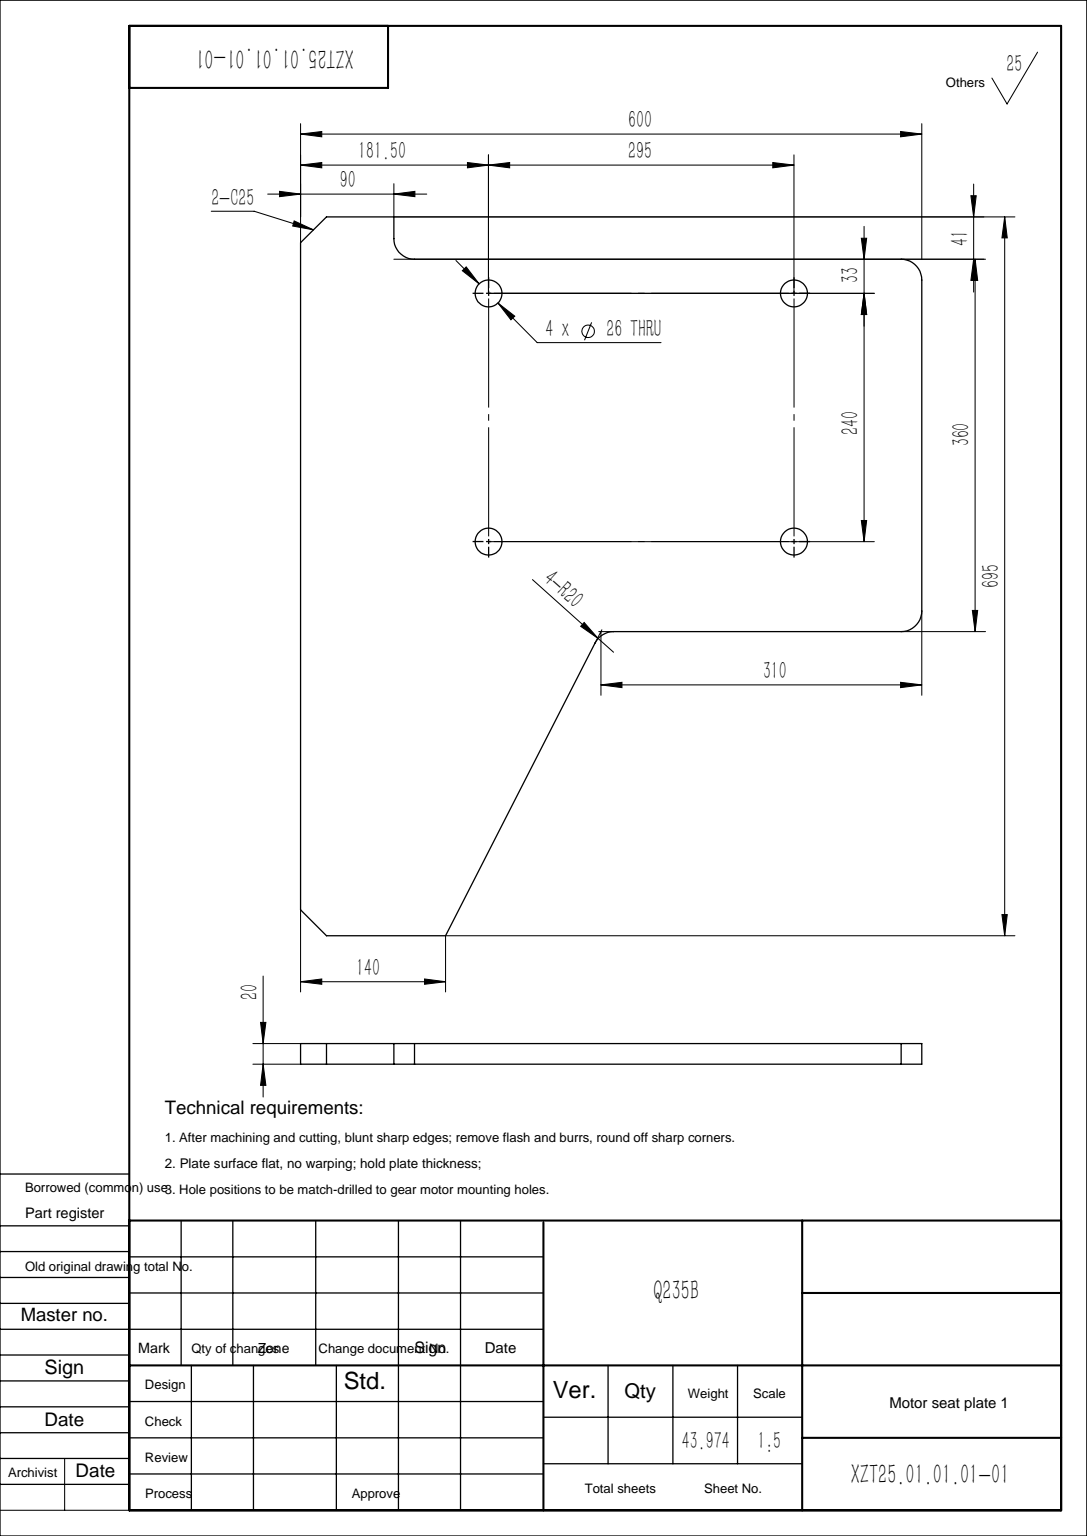
SolidWorks part; units mm, degrees
material "Q235B"
ref_plane "Front Plane" through (0, 0, 0) normal (0, 0, 1) x (1, 0, 0)
ref_plane "Top Plane" through (0, 0, 0) normal (0, 1, 0) x (1, 0, 0)
ref_plane "Right Plane" through (0, 0, 0) normal (1, 0, 0) x (0, 0, -1)
sketch "Sketch1" plane through (0, 0, 0) normal (0, 0, 1) x (1, 0, 0)
  line L0 (0, 0) -> (0, 695)
  line L1 (0, 695) -> (90, 695)
  line L2 (90, 695) -> (90, 654)
  line L3 (90, 654) -> (600, 654)
  line L4 (600, 654) -> (600, 294)
  line L5 (600, 294) -> (290, 294)
  line L6 (290, 294) -> (140, 0)
  line L7 (140, 0) -> (0, 0)
  dimension "D1" = 140
  dimension "D2" = 310
  dimension "D3" = 360
  dimension "D4" = 695
  dimension "D5" = 41
  dimension "D6" = 600
  dimension "D7" = 90
extrude "Boss-Extrude1" add sketch "Sketch1" along normal mid plane 20
chamfer "Chamfer1" distance 25 angle 45 2 edges at (0, 0, 0) (0, 695, 0)
fillet "Fillet1" radius 20 4 edges at (600, 294, 0) (600, 654, 0) (90, 654, 0) (290, 294, 0)
hole_wizard "Ø26 Diameter Hole1" positions "Sketch2" profile "Sketch3" hole size "Ø25.0" standard "GB" end condition up to next
sketch "Sketch2" plane through (0, 0, 10) normal (0, 0, 1) x (1, 0, 0)
  line L0 (181.5, 621) -> (181.5, 381) construction
  line L1 (0, 670) -> (0, 25) construction
  line L2 (580, 654) -> (110, 654) construction
  point P0 (181.5, 621)
  point P5 (476.5, 621)
  point P6 (476.5, 381)
  point P7 (181.5, 381)
  dimension "D3" = 240
  dimension "D4" = 181.5
  dimension "D5" = 33
  dimension "D6" = 295
  dimension "D1" = 2
  dimension "D2" = 2
sketch "Sketch3" plane through (181.5, 621, 10) normal (1, 0, 0) x (0, -1, 0)
  line L0 (0, 0) -> (0, 20)
  line L1 (0, 20) -> (13, 20)
  line L2 (13, 20) -> (13, 0)
  line L5 (13, 0) -> (0, 0)
  line L11 (0, -6.35) -> (0, 107.95) construction
  dimension "通孔孔直径" = 26
  dimension "通孔孔深度" = 20
